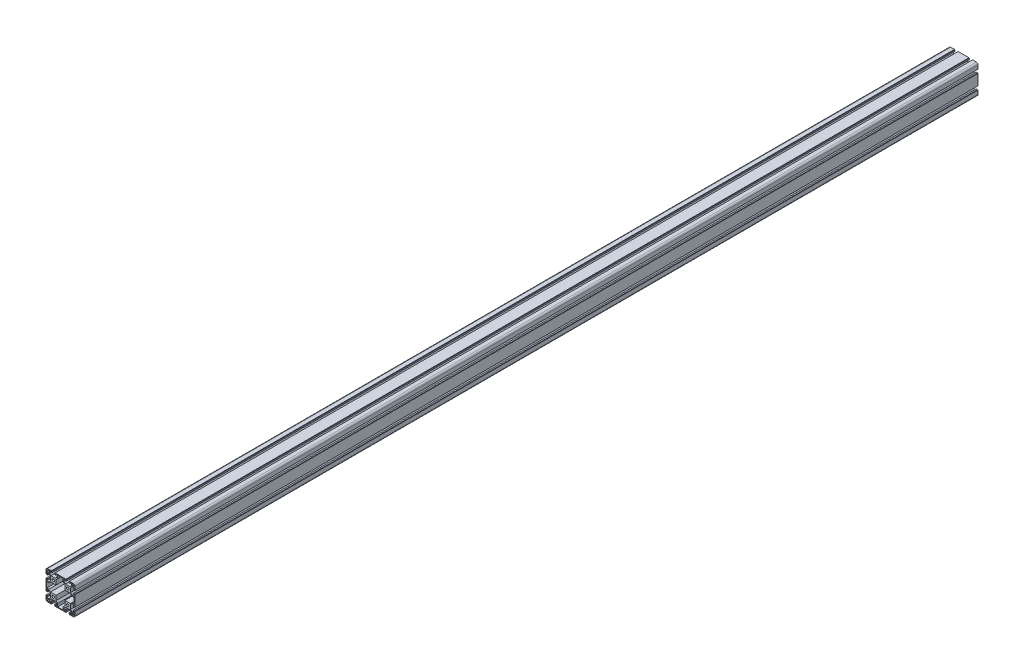
SolidWorks part; units mm, degrees
material "6061 合金"
ref_plane "前视基准面" through (0, 0, 0) normal (0, 0, 1) x (1, 0, 0)
ref_plane "上视基准面" through (0, 0, 0) normal (0, 1, 0) x (1, 0, 0)
ref_plane "右视基准面" through (0, 0, 0) normal (1, 0, 0) x (0, 0, -1)
sketch "草图1" plane through (0, 0, 0) normal (0, 0, 1) x (1, 0, 0)
  line L0 (0, 40) -> (0, 0) construction
  line L1 (-40, 40) -> (40, 40)
  line L2 (-40, 40) -> (-40, -40)
  line L3 (-40, -40) -> (40, -40)
  line L4 (40, 40) -> (40, -40)
  line L5 (0, 0) -> (-40, 0) construction
  dimension "D1" = 80
  dimension "D2" = 80
extrude "凸台-拉伸1" add sketch "草图1" along normal mid plane 2500
fillet "圆角1" radius 4.5 4 edges at (40, -40, 0) (40, 40, 0) (-40, -40, 0) (-40, 40, 0)
sketch "草图2" plane through (0, 0, -1250) normal (0, 0, -1) x (-1, 0, 0)
  line L0 (35.5, -40) -> (-35.5, -40) construction
  line L1 (-38, -31.7) -> (-31.7, -31.7)
  line L2 (-38, -31.7) -> (-38, -38)
  line L3 (-38, -38) -> (-31.7, -38)
  line L4 (-31.7, -31.7) -> (-31.7, -38)
  line L5 (-40, -35.5) -> (-40, 35.5) construction
  dimension "D1" = 6.3
  dimension "D2" = 6.3
  dimension "D3" = 2
  dimension "D4" = 2
extrude "切除-拉伸1" cut sketch "草图2" against normal through all
fillet "圆角2" radius 2.5 1 edges at (38, -38, 0)
hole_wizard "Ø6.8 (6.8) 直径孔1" positions "草图4" profile "草图5" hole size "Ø6.8" standard "Gb" end condition through all
sketch "草图4" plane through (0, 0, -1250) normal (0, 0, -1) x (-1, 0, 0)
  line L0 (-40, -35.5) -> (-40, 35.5) construction
  line L1 (35.5, -40) -> (-35.5, -40) construction
  point P0 (-20, -20)
  dimension "D1" = 20
  dimension "D2" = 20
sketch "草图5" plane through (20, -20, -1250) normal (1, 0, 0) x (0, 1, 0)
  line L0 (0, 0) -> (0, 2500)
  line L1 (0, 2500) -> (3.25, 2500)
  line L2 (3.25, 2500) -> (3.25, 0)
  line L5 (3.25, 0) -> (0, 0)
  line L11 (0, -6.35) -> (0, 107.95) construction
  dimension "通孔孔直径" = 6.5
  dimension "通孔孔深度" = 2500
sketch "草图6" plane through (0, 0, -1250) normal (0, 0, -1) x (-1, 0, 0)
  line L0 (-25, -43.6805) -> (-25, -39)
  line L1 (-25, -39) -> (-24.1, -39)
  line L2 (-24.1, -39) -> (-24.1, -35.5)
  line L3 (-24.1, -35.5) -> (-26.5, -35.5)
  line L4 (-26.5, -35.5) -> (-26.5, -38)
  line L5 (-26.5, -38) -> (-30.25, -38)
  line L6 (-30.25, -38) -> (-30.25, -32)
  line L7 (-30.25, -32) -> (-26, -27.7)
  line L8 (-26, -27.7) -> (-14, -27.7)
  line L9 (-14, -27.7) -> (-9.75, -32)
  line L10 (-9.75, -32) -> (-9.75, -38)
  line L11 (-9.75, -38) -> (-13.5, -38)
  line L12 (-13.5, -38) -> (-13.5, -35.5)
  line L13 (-13.5, -35.5) -> (-15.9, -35.5)
  line L14 (-15.9, -35.5) -> (-15.9, -39)
  line L15 (-15.9, -39) -> (-15, -39)
  line L16 (-15, -39) -> (-15, -43.6805)
  line L17 (-25, -43.6805) -> (-15, -43.6805)
  line L18 (-20, -20) -> (-20, -54.4042) construction
  line L20 (35.5, -40) -> (-35.5, -40) construction
  dimension "D1" = 12.3
  dimension "D2" = 2
  dimension "D3" = 4.5
  dimension "D4" = 8.2
  dimension "D5" = 1
  dimension "D6" = 10
  dimension "D7" = 13
  dimension "D8" = 20.5
  dimension "D9" = 12
  dimension "D10" = 6
extrude "切除-拉伸2" cut sketch "草图6" against normal through all
ref_plane "基准面1" through (0, 0, 0) normal (-0.7071, -0.7071, 0) x (-0.7071, 0.7071, 0)
mirror "镜向1" about plane through (0, 0, 0) normal (-0.7071, -0.7071, 0) of "切除-拉伸2"
mirror "镜向2" about plane through (0, 0, 0) normal (0, 1, 0) of "Ø6.8 (6.8) 直径孔1", "镜向1", "切除-拉伸1", "切除-拉伸2"
mirror "镜向3" about plane through (0, 0, 0) normal (1, 0, 0) of "镜向2", "切除-拉伸1", "Ø6.8 (6.8) 直径孔1", "切除-拉伸2", "镜向1"
sketch "草图7" plane through (0, 0, -1250) normal (0, 0, -1) x (-1, 0, 0)
  line L0 (-7.75, 38) -> (-7.75, 29.6186)
  line L1 (-7.75, 29.6186) -> (-12.2, 25.1686)
  line L2 (-12.2, 25.1686) -> (-12.2, 12.2)
  line L3 (-12.2, 12.2) -> (-27.6639, 12.2)
  line L4 (-27.6639, 12.2) -> (-32.1139, 7.75)
  line L5 (-32.1139, 7.75) -> (-38, 7.75)
  line L6 (-38, 7.75) -> (-38, -7.75)
  line L7 (-38, -7.75) -> (-32.1139, -7.75)
  line L8 (-32.1139, -7.75) -> (-27.6639, -12.2)
  line L9 (-27.6639, -12.2) -> (-12.2, -12.2)
  line L10 (-12.2, -12.2) -> (-12.2, -25.1686)
  line L11 (-12.2, -25.1686) -> (-7.75, -29.6186)
  line L12 (-7.75, -29.6186) -> (-7.75, -38)
  line L13 (-7.75, -38) -> (7.75, -38)
  line L14 (7.75, -38) -> (7.75, -29.6186)
  line L15 (7.75, -29.6186) -> (12.2, -25.1686)
  line L16 (12.2, -25.1686) -> (12.2, -12.2)
  line L17 (12.2, -12.2) -> (27.6639, -12.2)
  line L18 (27.6639, -12.2) -> (32.1139, -7.75)
  line L19 (32.1139, -7.75) -> (38, -7.75)
  line L20 (38, -7.75) -> (38, 7.75)
  line L21 (38, 7.75) -> (32.1139, 7.75)
  line L22 (32.1139, 7.75) -> (27.6639, 12.2)
  line L23 (27.6639, 12.2) -> (12.2, 12.2)
  line L24 (12.2, 12.2) -> (12.2, 25.1686)
  line L25 (12.2, 25.1686) -> (7.75, 29.6186)
  line L26 (7.75, 29.6186) -> (7.75, 38)
  line L27 (7.75, 38) -> (-7.75, 38)
  line L28 (0, 40) -> (0, -53.8168) construction
  line L29 (-15, 40) -> (15, 40) construction
  line L30 (-40, 0) -> (64.558, 0) construction
  line L31 (-40, -15) -> (-40, 15) construction
  line L32 (40, 15) -> (40, -15) construction
  line L33 (15, -40) -> (-15, -40) construction
  line L34 (14, -27.7) -> (26, -27.7) construction
  line L35 (27.7, -14) -> (27.7, -26) construction
  line L36 (9.75, -38) -> (9.75, -32) construction
  line L39 (38, -9.75) -> (32, -9.75) construction
  dimension "D1" = 2
  dimension "D2" = 2
  dimension "D3" = 15.5
  dimension "D4" = 15.5
  dimension "D5" = 2
  dimension "D6" = 2
extrude "切除-拉伸3" cut sketch "草图7" against normal through all
sketch "草图8" plane through (40, 0, 0) normal (1, 0, 0) x (0, 0, -1)
  line L0 (-1250, 40) -> (1250, 40) construction
  line L1 (-450, 40) -> (-355, 40)
  line L2 (-450, 40) -> (-450, -40)
  line L3 (-450, -40) -> (-355, -40)
  line L4 (-355, 40) -> (-355, -40)
  line L5 (1250, -40) -> (-1250, -40) construction
  line L6 (-1250, -15) -> (-1250, 15) construction
  dimension "D1" = 95
  dimension "D2" = 800
hole_wizard "M8 螺纹孔1" positions "草图10" profile "草图9" tap size "M8" standard "ISO"
sketch "草图10" plane through (0, 0, -1250) normal (0, 0, -1) x (-1, 0, 0)
  point P0 (-20, 20)
  point P3 (20, 20)
  point P6 (20, -20)
  point P9 (-20, -20)
cosmetic thread "孔螺蚊线1" parameters "D1"=10, "D2"=8
cosmetic thread "孔螺蚊线2" parameters "D1"=10, "D2"=8
cosmetic thread "孔螺蚊线3" parameters "D1"=10, "D2"=8
cosmetic thread "孔螺蚊线4" parameters "D1"=10, "D2"=8
sketch "草图9" plane through (20, 20, -1250) normal (1, 0, 0) x (0, 1, 0)
  line L0 (0, 0) -> (0, 15.7929)
  line L1 (0, 15.7929) -> (3.4, 13.75)
  line L2 (3.4, 13.75) -> (3.4, 0)
  line L5 (3.4, 0) -> (0, 0)
  line L10 (0, 15.7929) -> (-3.4, 13.75) construction
  line L11 (0, -6.35) -> (0, 107.95) construction
  dimension "螺纹孔钻头直径" = 6.8
  dimension "螺纹孔钻头深度" = 13.75
  dimension "导头角度" = 118
hole_wizard "M8 螺纹孔2" positions "草图13" profile "草图12" tap size "M8" standard "ISO"
sketch "草图13" plane through (0, 0, 1250) normal (0, 0, 1) x (1, 0, 0)
  point P0 (-20, 20)
  point P3 (20, 20)
  point P6 (20, -20)
  point P9 (-20, -20)
sketch "草图12" plane through (-20, 20, 1250) normal (1, 0, 0) x (0, -1, 0)
  line L0 (0, 0) -> (0, 15.7929)
  line L1 (0, 15.7929) -> (3.4, 13.75)
  line L2 (3.4, 13.75) -> (3.4, 0)
  line L5 (3.4, 0) -> (0, 0)
  line L10 (0, 15.7929) -> (-3.4, 13.75) construction
  line L11 (0, -6.35) -> (0, 107.95) construction
  dimension "螺纹孔钻头直径" = 6.8
  dimension "螺纹孔钻头深度" = 13.75
  dimension "导头角度" = 118
cosmetic thread "孔螺蚊线5" parameters "D1"=0, "D2"=7.8
cosmetic thread "孔螺蚊线6" parameters "D1"=0, "D2"=7.8
cosmetic thread "孔螺蚊线7" parameters "D1"=0, "D2"=7.8
cosmetic thread "孔螺蚊线8" parameters "D1"=0, "D2"=7.8
